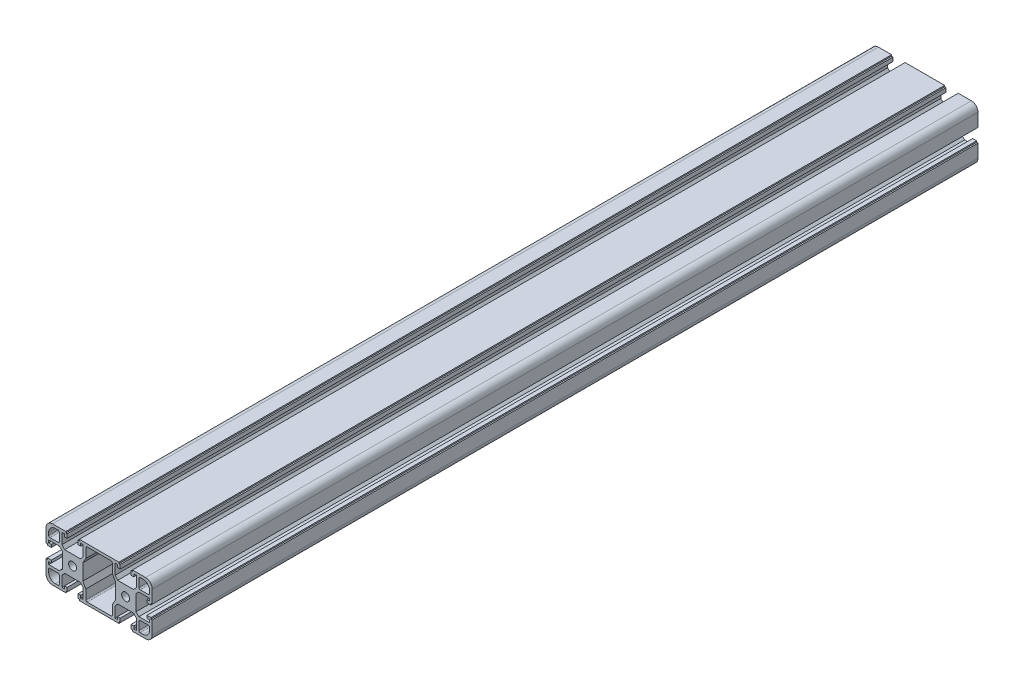
SolidWorks part; units mm, degrees
ref_plane "前视基准面" through (0, 0, 0) normal (0, 0, 1) x (1, 0, 0)
ref_plane "上视基准面" through (0, 0, 0) normal (0, 1, 0) x (1, 0, 0)
ref_plane "右视基准面" through (0, 0, 0) normal (1, 0, 0) x (0, 0, -1)
sketch "草图1" plane through (0, 0, 0) normal (0, 0, 1) x (1, 0, 0)
  line L0 (0, 0) -> (0, 24.5989) construction
  line L1 (-5.1, 20) -> (-5.1, 19)
  line L2 (-20, 20) -> (-5.1, 20)
  line L3 (-20, 20) -> (-20, 5.1)
  line L4 (-20, -20) -> (-5.1, -20)
  line L5 (0, 0) -> (20, 0) construction
  line L6 (7.7, 6) -> (10, 10)
  line L7 (-5.1, 19) -> (-4.1, 19)
  line L8 (-4.1, 19) -> (-4.1, 16)
  line L9 (-4.1, 16) -> (-6.1, 16)
  line L10 (-6.1, 16) -> (-6.1, 18)
  line L11 (-6.1, 18) -> (-8, 18)
  line L12 (-8, 18) -> (-8, 10)
  line L13 (-8, 10) -> (-6, 7.7)
  line L14 (-6, 7.7) -> (6, 7.7)
  line L15 (8, 10) -> (6, 7.7)
  line L16 (8, 18) -> (8, 10)
  line L17 (6.1, 18) -> (8, 18)
  line L18 (6.1, 16) -> (6.1, 18)
  line L19 (4.1, 16) -> (6.1, 16)
  line L20 (4.1, 19) -> (4.1, 16)
  line L21 (5.1, 19) -> (4.1, 19)
  line L22 (5.1, 20) -> (5.1, 19)
  line L23 (5.1, -20) -> (5.1, -19)
  line L24 (5.1, -19) -> (4.1, -19)
  line L25 (4.1, -19) -> (4.1, -16)
  line L26 (4.1, -16) -> (6.1, -16)
  line L27 (6.1, -16) -> (6.1, -18)
  line L28 (6.1, -18) -> (8, -18)
  line L29 (8, -18) -> (8, -10)
  line L30 (8, -10) -> (6, -7.7)
  line L31 (-6, -7.7) -> (6, -7.7)
  line L32 (-8, -10) -> (-6, -7.7)
  line L33 (-8, -18) -> (-8, -10)
  line L34 (-6.1, -18) -> (-8, -18)
  line L35 (-6.1, -16) -> (-6.1, -18)
  line L36 (-4.1, -16) -> (-6.1, -16)
  line L37 (-4.1, -19) -> (-4.1, -16)
  line L38 (-5.1, -19) -> (-4.1, -19)
  line L39 (-5.1, -20) -> (-5.1, -19)
  line L40 (7.7, -6) -> (10, -10)
  line L41 (30, 10) -> (32.3, 6)
  line L42 (30, -10) -> (32.3, -6)
  line L55 (7.7, 6) -> (7.7, -6)
  line L57 (-19, -5.1) -> (-19, -4.1)
  line L58 (-7.7, 6) -> (-7.7, -6)
  line L59 (-10, 8) -> (-7.7, 6)
  line L60 (-18, 6.1) -> (-18, 8)
  line L61 (-19, 4.1) -> (-16, 4.1)
  line L62 (-16, 4.1) -> (-16, 6.1)
  line L63 (-20, 5.1) -> (-19, 5.1)
  line L64 (-18, -6.1) -> (-18, -8)
  line L65 (-16, -4.1) -> (-16, -6.1)
  line L66 (-16, -6.1) -> (-18, -6.1)
  line L67 (-16, 6.1) -> (-18, 6.1)
  line L68 (-10, -8) -> (-7.7, -6)
  line L69 (-19, 5.1) -> (-19, 4.1)
  line L70 (-18, -8) -> (-10, -8)
  line L71 (-18, 8) -> (-10, 8)
  line L72 (-20, -5.1) -> (-19, -5.1)
  line L73 (-19, -4.1) -> (-16, -4.1)
  line L74 (5.1, 20) -> (34.9, 20)
  line L75 (-20, -5.1) -> (-20, -20)
  line L76 (5.1, -20) -> (34.9, -20)
  line L78 (10, 18) -> (10, 10)
  line L79 (-18, 18) -> (-10, 18)
  line L80 (-18, 18) -> (-18, 10)
  line L81 (-18, 10) -> (-10, 10)
  line L82 (-10, 18) -> (-10, 10)
  line L85 (30, 18) -> (10, 18)
  line L89 (10, -18) -> (10, -10)
  line L90 (-10, -18) -> (-10, -10)
  line L91 (-18, -10) -> (-10, -10)
  line L92 (-18, -18) -> (-18, -10)
  line L93 (-18, -18) -> (-10, -18)
  line L94 (20, 0) -> (20, 30.8422) construction
  line L95 (58, -18) -> (50, -18)
  line L96 (58, -18) -> (58, -10)
  line L97 (58, -10) -> (50, -10)
  line L98 (50, -18) -> (50, -10)
  line L99 (30, -18) -> (30, -10)
  line L102 (10, -18) -> (30, -18)
  line L106 (50, 18) -> (50, 10)
  line L107 (58, 10) -> (50, 10)
  line L108 (58, 18) -> (58, 10)
  line L109 (58, 18) -> (50, 18)
  line L110 (30, 18) -> (30, 10)
  line L111 (60, -5.1) -> (60, -20)
  line L112 (59, -4.1) -> (56, -4.1)
  line L113 (60, -5.1) -> (59, -5.1)
  line L114 (58, 8) -> (50, 8)
  line L115 (58, -8) -> (50, -8)
  line L116 (59, 5.1) -> (59, 4.1)
  line L117 (50, -8) -> (47.7, -6)
  line L118 (56, 6.1) -> (58, 6.1)
  line L119 (56, -6.1) -> (58, -6.1)
  line L120 (56, -4.1) -> (56, -6.1)
  line L121 (58, -6.1) -> (58, -8)
  line L122 (60, 5.1) -> (59, 5.1)
  line L123 (56, 4.1) -> (56, 6.1)
  line L124 (59, 4.1) -> (56, 4.1)
  line L125 (58, 6.1) -> (58, 8)
  line L126 (50, 8) -> (47.7, 6)
  line L127 (47.7, 6) -> (47.7, -6)
  line L128 (59, -5.1) -> (59, -4.1)
  line L130 (32.3, 6) -> (32.3, -6)
  line L144 (45.1, -20) -> (45.1, -19)
  line L145 (45.1, -19) -> (44.1, -19)
  line L146 (44.1, -19) -> (44.1, -16)
  line L147 (44.1, -16) -> (46.1, -16)
  line L148 (46.1, -16) -> (46.1, -18)
  line L149 (46.1, -18) -> (48, -18)
  line L150 (48, -18) -> (48, -10)
  line L151 (48, -10) -> (46, -7.7)
  line L152 (46, -7.7) -> (34, -7.7)
  line L153 (32, -10) -> (34, -7.7)
  line L154 (32, -18) -> (32, -10)
  line L155 (33.9, -18) -> (32, -18)
  line L156 (33.9, -16) -> (33.9, -18)
  line L157 (35.9, -16) -> (33.9, -16)
  line L158 (35.9, -19) -> (35.9, -16)
  line L159 (34.9, -19) -> (35.9, -19)
  line L160 (34.9, -20) -> (34.9, -19)
  line L161 (34.9, 20) -> (34.9, 19)
  line L162 (34.9, 19) -> (35.9, 19)
  line L163 (35.9, 19) -> (35.9, 16)
  line L164 (35.9, 16) -> (33.9, 16)
  line L165 (33.9, 16) -> (33.9, 18)
  line L166 (33.9, 18) -> (32, 18)
  line L167 (32, 18) -> (32, 10)
  line L168 (32, 10) -> (34, 7.7)
  line L169 (46, 7.7) -> (34, 7.7)
  line L170 (48, 10) -> (46, 7.7)
  line L171 (48, 18) -> (48, 10)
  line L172 (46.1, 18) -> (48, 18)
  line L173 (46.1, 16) -> (46.1, 18)
  line L174 (44.1, 16) -> (46.1, 16)
  line L175 (44.1, 19) -> (44.1, 16)
  line L176 (45.1, 19) -> (44.1, 19)
  line L177 (60, -20) -> (45.1, -20)
  line L178 (60, 20) -> (60, 5.1)
  line L179 (60, 20) -> (45.1, 20)
  line L180 (45.1, 20) -> (45.1, 19)
  circle A0 centre (0, 0) radius 3
  circle A1 centre (40, 0) radius 3
  point P19 (0, 7.7)
  point P27 (0, -7.7)
  point P102 (40, -7.7)
  point P103 (40, 7.7)
  dimension "D12" = 10
  dimension "D23" = 6
  dimension "D2" = 40
  dimension "D3" = 8.2
  dimension "D4" = 10.2
  dimension "D5" = 1
  dimension "D6" = 2
  dimension "D7" = 4
  dimension "D8" = 2
  dimension "D9" = 16
  dimension "D10" = 12.3
  dimension "D11" = 12
  dimension "D13" = 20
  dimension "D14" = 80
  dimension "D15" = 2
  dimension "D16" = 10
  dimension "D17" = 8.2
  dimension "D18" = 10.2
  dimension "D19" = 12.2
  dimension "D20" = 1
  dimension "D21" = 4
  dimension "D22" = 12
  dimension "D24" = 2
  dimension "D25" = 2
  dimension "D26" = 12.3
  dimension "D27" = 10
extrude "拉伸1" add sketch "草图1" along normal mid plane 647
fillet "圆角1" radius 5 8 edges at (-20, -20, 0) (-20, 20, 0) (-18, -18, 0) (-18, 18, 0) (60, -20, 0) (60, 20, 0) (58, -18, 0) (58, 18, 0)
fillet "圆角2" radius 1 16 edges at (-10, -10, 0) (-18, -10, 0) (-10, 18, 0) (10, 18, 0) (-10, -18, 0) (-10, 10, 0) (-18, 10, 0) (50, 18, 0) (50, 10, 0) (58, 10, 0) (58, -10, 0) (50, -10, 0) (50, -18, 0) (30, 18, 0) (30, -18, 0) (10, -18, 0)
sketch "草图4" plane through (0, 0, -323.5) normal (0, 0, -1) x (-1, 0, 0)
  line L112 (-60, -5.1) -> (-60, -15)
  line L113 (-55, -20) -> (-45.1, -20)
  line L114 (-45.1, -20) -> (-45.1, -19)
  line L115 (-45.1, -19) -> (-44.1, -19)
  line L116 (-44.1, -19) -> (-44.1, -16)
  line L117 (-44.1, -16) -> (-46.1, -16)
  line L118 (-46.1, -16) -> (-46.1, -18)
  line L119 (-46.1, -18) -> (-48, -18)
  line L120 (-48, -18) -> (-48, -10)
  line L121 (-48, -10) -> (-46, -7.7)
  line L122 (-46, -7.7) -> (-34, -7.7)
  line L123 (-34, -7.7) -> (-32, -10)
  line L124 (-32, -10) -> (-32, -18)
  line L125 (-32, -18) -> (-33.9, -18)
  line L126 (-33.9, -18) -> (-33.9, -16)
  line L127 (-33.9, -16) -> (-35.9, -16)
  line L128 (-35.9, -16) -> (-35.9, -19)
  line L129 (-35.9, -19) -> (-34.9, -19)
  line L130 (-34.9, -19) -> (-34.9, -20)
  line L131 (-34.9, -20) -> (-5.1, -20)
  line L132 (-5.1, -20) -> (-5.1, -19)
  line L133 (-5.1, -19) -> (-4.1, -19)
  line L134 (-4.1, -19) -> (-4.1, -16)
  line L135 (-4.1, -16) -> (-6.1, -16)
  line L136 (-6.1, -16) -> (-6.1, -18)
  line L137 (-6.1, -18) -> (-8, -18)
  line L138 (-8, -18) -> (-8, -10)
  line L139 (-8, -10) -> (-6, -7.7)
  line L140 (-6, -7.7) -> (6, -7.7)
  line L141 (6, -7.7) -> (8, -10)
  line L142 (8, -10) -> (8, -18)
  line L143 (8, -18) -> (6.1, -18)
  line L144 (6.1, -18) -> (6.1, -16)
  line L145 (6.1, -16) -> (4.1, -16)
  line L146 (4.1, -16) -> (4.1, -19)
  line L147 (4.1, -19) -> (5.1, -19)
  line L148 (5.1, -19) -> (5.1, -20)
  line L149 (5.1, -20) -> (15, -20)
  line L150 (20, -15) -> (20, -5.1)
  line L151 (20, -5.1) -> (19, -5.1)
  line L152 (19, -5.1) -> (19, -4.1)
  line L153 (19, -4.1) -> (16, -4.1)
  line L154 (16, -4.1) -> (16, -6.1)
  line L155 (16, -6.1) -> (18, -6.1)
  line L156 (18, -6.1) -> (18, -8)
  line L157 (18, -8) -> (10, -8)
  line L158 (10, -8) -> (7.7, -6)
  line L159 (7.7, -6) -> (7.7, 6)
  line L160 (7.7, 6) -> (10, 8)
  line L161 (10, 8) -> (18, 8)
  line L162 (18, 8) -> (18, 6.1)
  line L163 (18, 6.1) -> (16, 6.1)
  line L164 (16, 6.1) -> (16, 4.1)
  line L165 (16, 4.1) -> (19, 4.1)
  line L166 (19, 4.1) -> (19, 5.1)
  line L167 (19, 5.1) -> (20, 5.1)
  line L168 (20, 5.1) -> (20, 15)
  line L169 (15, 20) -> (5.1, 20)
  line L170 (5.1, 20) -> (5.1, 19)
  line L171 (5.1, 19) -> (4.1, 19)
  line L172 (4.1, 19) -> (4.1, 16)
  line L173 (4.1, 16) -> (6.1, 16)
  line L174 (6.1, 16) -> (6.1, 18)
  line L175 (6.1, 18) -> (8, 18)
  line L176 (8, 18) -> (8, 10)
  line L177 (8, 10) -> (6, 7.7)
  line L178 (6, 7.7) -> (-6, 7.7)
  line L179 (-6, 7.7) -> (-8, 10)
  line L180 (-8, 10) -> (-8, 18)
  line L181 (-8, 18) -> (-6.1, 18)
  line L182 (-6.1, 18) -> (-6.1, 16)
  line L183 (-6.1, 16) -> (-4.1, 16)
  line L184 (-4.1, 16) -> (-4.1, 19)
  line L185 (-4.1, 19) -> (-5.1, 19)
  line L186 (-5.1, 19) -> (-5.1, 20)
  line L187 (-5.1, 20) -> (-34.9, 20)
  line L188 (-34.9, 20) -> (-34.9, 19)
  line L189 (-34.9, 19) -> (-35.9, 19)
  line L190 (-35.9, 19) -> (-35.9, 16)
  line L191 (-35.9, 16) -> (-33.9, 16)
  line L192 (-33.9, 16) -> (-33.9, 18)
  line L193 (-33.9, 18) -> (-32, 18)
  line L194 (-32, 18) -> (-32, 10)
  line L195 (-32, 10) -> (-34, 7.7)
  line L196 (-34, 7.7) -> (-46, 7.7)
  line L197 (-46, 7.7) -> (-48, 10)
  line L198 (-48, 10) -> (-48, 18)
  line L199 (-48, 18) -> (-46.1, 18)
  line L200 (-46.1, 18) -> (-46.1, 16)
  line L201 (-46.1, 16) -> (-44.1, 16)
  line L202 (-44.1, 16) -> (-44.1, 19)
  line L203 (-44.1, 19) -> (-45.1, 19)
  line L204 (-45.1, 19) -> (-45.1, 20)
  line L205 (-45.1, 20) -> (-55, 20)
  line L206 (-60, 15) -> (-60, 5.1)
  line L207 (-60, 5.1) -> (-59, 5.1)
  line L208 (-59, 5.1) -> (-59, 4.1)
  line L209 (-59, 4.1) -> (-56, 4.1)
  line L210 (-56, 4.1) -> (-56, 6.1)
  line L211 (-56, 6.1) -> (-58, 6.1)
  line L212 (-58, 6.1) -> (-58, 8)
  line L213 (-58, 8) -> (-50, 8)
  line L214 (-50, 8) -> (-47.7, 6)
  line L215 (-47.7, 6) -> (-47.7, -6)
  line L216 (-47.7, -6) -> (-50, -8)
  line L217 (-50, -8) -> (-58, -8)
  line L218 (-58, -8) -> (-58, -6.1)
  line L219 (-58, -6.1) -> (-56, -6.1)
  line L220 (-56, -6.1) -> (-56, -4.1)
  line L221 (-56, -4.1) -> (-59, -4.1)
  line L222 (-59, -4.1) -> (-59, -5.1)
  line L223 (-59, -5.1) -> (-60, -5.1)
  line L224 (-60, -5.1) -> (-60, -15)
  line L225 (-55, -20) -> (-45.1, -20)
  line L226 (-45.1, -20) -> (-45.1, -19)
  line L227 (-45.1, -19) -> (-44.1, -19)
  line L228 (-44.1, -19) -> (-44.1, -16)
  line L229 (-44.1, -16) -> (-46.1, -16)
  line L230 (-46.1, -16) -> (-46.1, -18)
  line L231 (-46.1, -18) -> (-48, -18)
  line L232 (-48, -18) -> (-48, -10)
  line L233 (-48, -10) -> (-46, -7.7)
  line L234 (-46, -7.7) -> (-34, -7.7)
  line L235 (-34, -7.7) -> (-32, -10)
  line L236 (-32, -10) -> (-32, -18)
  line L237 (-32, -18) -> (-33.9, -18)
  line L238 (-33.9, -18) -> (-33.9, -16)
  line L239 (-33.9, -16) -> (-35.9, -16)
  line L240 (-35.9, -16) -> (-35.9, -19)
  line L241 (-35.9, -19) -> (-34.9, -19)
  line L242 (-34.9, -19) -> (-34.9, -20)
  line L243 (-34.9, -20) -> (-5.1, -20)
  line L244 (-5.1, -20) -> (-5.1, -19)
  line L245 (-5.1, -19) -> (-4.1, -19)
  line L246 (-4.1, -19) -> (-4.1, -16)
  line L247 (-4.1, -16) -> (-6.1, -16)
  line L248 (-6.1, -16) -> (-6.1, -18)
  line L249 (-6.1, -18) -> (-8, -18)
  line L250 (-8, -18) -> (-8, -10)
  line L251 (-8, -10) -> (-6, -7.7)
  line L252 (-6, -7.7) -> (6, -7.7)
  line L253 (6, -7.7) -> (8, -10)
  line L254 (8, -10) -> (8, -18)
  line L255 (8, -18) -> (6.1, -18)
  line L256 (6.1, -18) -> (6.1, -16)
  line L257 (6.1, -16) -> (4.1, -16)
  line L258 (4.1, -16) -> (4.1, -19)
  line L259 (4.1, -19) -> (5.1, -19)
  line L260 (5.1, -19) -> (5.1, -20)
  line L261 (5.1, -20) -> (15, -20)
  line L262 (20, -15) -> (20, -5.1)
  line L263 (20, -5.1) -> (19, -5.1)
  line L264 (19, -5.1) -> (19, -4.1)
  line L265 (19, -4.1) -> (16, -4.1)
  line L266 (16, -4.1) -> (16, -6.1)
  line L267 (16, -6.1) -> (18, -6.1)
  line L268 (18, -6.1) -> (18, -8)
  line L269 (18, -8) -> (10, -8)
  line L270 (10, -8) -> (7.7, -6)
  line L271 (7.7, -6) -> (7.7, 6)
  line L272 (7.7, 6) -> (10, 8)
  line L273 (10, 8) -> (18, 8)
  line L274 (18, 8) -> (18, 6.1)
  line L275 (18, 6.1) -> (16, 6.1)
  line L276 (16, 6.1) -> (16, 4.1)
  line L277 (16, 4.1) -> (19, 4.1)
  line L278 (19, 4.1) -> (19, 5.1)
  line L279 (19, 5.1) -> (20, 5.1)
  line L280 (20, 5.1) -> (20, 15)
  line L281 (15, 20) -> (5.1, 20)
  line L282 (5.1, 20) -> (5.1, 19)
  line L283 (5.1, 19) -> (4.1, 19)
  line L284 (4.1, 19) -> (4.1, 16)
  line L285 (4.1, 16) -> (6.1, 16)
  line L286 (6.1, 16) -> (6.1, 18)
  line L287 (6.1, 18) -> (8, 18)
  line L288 (8, 18) -> (8, 10)
  line L289 (8, 10) -> (6, 7.7)
  line L290 (6, 7.7) -> (-6, 7.7)
  line L291 (-6, 7.7) -> (-8, 10)
  line L292 (-8, 10) -> (-8, 18)
  line L293 (-8, 18) -> (-6.1, 18)
  line L294 (-6.1, 18) -> (-6.1, 16)
  line L295 (-6.1, 16) -> (-4.1, 16)
  line L296 (-4.1, 16) -> (-4.1, 19)
  line L297 (-4.1, 19) -> (-5.1, 19)
  line L298 (-5.1, 19) -> (-5.1, 20)
  line L299 (-5.1, 20) -> (-34.9, 20)
  line L300 (-34.9, 20) -> (-34.9, 19)
  line L301 (-34.9, 19) -> (-35.9, 19)
  line L302 (-35.9, 19) -> (-35.9, 16)
  line L303 (-35.9, 16) -> (-33.9, 16)
  line L304 (-33.9, 16) -> (-33.9, 18)
  line L305 (-33.9, 18) -> (-32, 18)
  line L306 (-32, 18) -> (-32, 10)
  line L307 (-32, 10) -> (-34, 7.7)
  line L308 (-34, 7.7) -> (-46, 7.7)
  line L309 (-46, 7.7) -> (-48, 10)
  line L310 (-48, 10) -> (-48, 18)
  line L311 (-48, 18) -> (-46.1, 18)
  line L312 (-46.1, 18) -> (-46.1, 16)
  line L313 (-46.1, 16) -> (-44.1, 16)
  line L314 (-44.1, 16) -> (-44.1, 19)
  line L315 (-44.1, 19) -> (-45.1, 19)
  line L316 (-45.1, 19) -> (-45.1, 20)
  line L317 (-45.1, 20) -> (-55, 20)
  line L318 (-60, 15) -> (-60, 5.1)
  line L319 (-60, 5.1) -> (-59, 5.1)
  line L320 (-59, 5.1) -> (-59, 4.1)
  line L321 (-59, 4.1) -> (-56, 4.1)
  line L322 (-56, 4.1) -> (-56, 6.1)
  line L323 (-56, 6.1) -> (-58, 6.1)
  line L324 (-58, 6.1) -> (-58, 8)
  line L325 (-58, 8) -> (-50, 8)
  line L326 (-50, 8) -> (-47.7, 6)
  line L327 (-47.7, 6) -> (-47.7, -6)
  line L328 (-47.7, -6) -> (-50, -8)
  line L329 (-50, -8) -> (-58, -8)
  line L330 (-58, -8) -> (-58, -6.1)
  line L331 (-58, -6.1) -> (-56, -6.1)
  line L332 (-56, -6.1) -> (-56, -4.1)
  line L333 (-56, -4.1) -> (-59, -4.1)
  line L334 (-59, -4.1) -> (-59, -5.1)
  line L335 (-59, -5.1) -> (-60, -5.1)
  arc A4 (-60, -15) -> (-55, -20) centre (-55, -15) ccw
  arc A5 (15, -20) -> (20, -15) centre (15, -15) ccw
  arc A6 (20, 15) -> (15, 20) centre (15, 15) ccw
  arc A7 (-55, 20) -> (-60, 15) centre (-55, 15) ccw
  arc A8 (-60, -15) -> (-55, -20) centre (-55, -15) ccw
  arc A9 (15, -20) -> (20, -15) centre (15, -15) ccw
  arc A10 (20, 15) -> (15, 20) centre (15, 15) ccw
  arc A11 (-55, 20) -> (-60, 15) centre (-55, 15) ccw
  dimension "D1" = 0
extrude "切除-拉伸1" cut sketch "草图4" against normal blind 25
